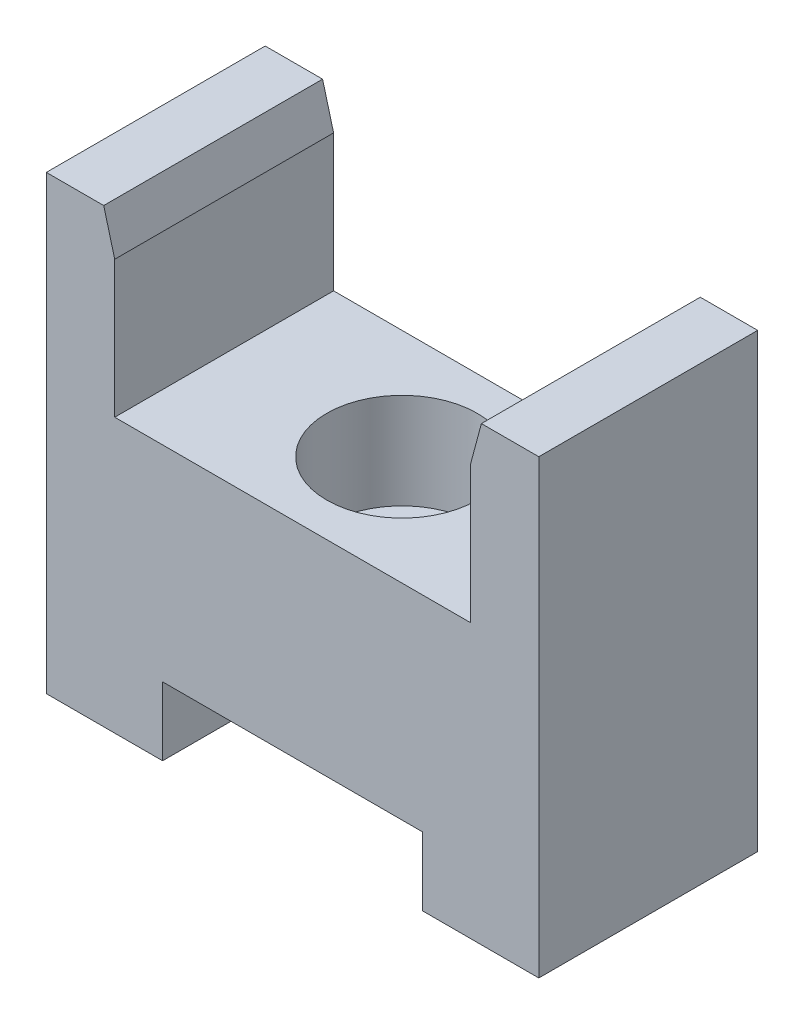
SolidWorks part; units mm, degrees
material "AISI 1045 钢，冷拔"
ref_plane "Front Plane" through (0, 0, 0) normal (0, 0, 1) x (1, 0, 0)
ref_plane "Top Plane" through (0, 0, 0) normal (0, 1, 0) x (1, 0, 0)
ref_plane "Right Plane" through (0, 0, 0) normal (1, 0, 0) x (0, 0, -1)
sketch "Sketch1" plane through (0, 0, 0) normal (0, 0, 1) x (1, 0, 0)
  line L0 (0, 33) -> (0, 0)
  line L1 (0, 0) -> (8.5, 0)
  line L2 (8.5, 0) -> (8.5, 5)
  line L3 (8.5, 5) -> (27.5, 5)
  line L4 (27.5, 5) -> (27.5, 0)
  line L5 (27.5, 0) -> (36, 0)
  line L6 (36, 0) -> (36, 33)
  line L10 (0, 33) -> (4.1962, 33)
  line L11 (4.1962, 33) -> (5, 30)
  line L12 (5, 30) -> (5, 20)
  line L13 (5, 20) -> (31, 20)
  line L14 (31, 20) -> (31, 30)
  line L15 (31, 30) -> (31.8038, 33)
  line L16 (31.8038, 33) -> (36, 33)
  dimension "D1" = 33
  dimension "D2" = 8.5
  dimension "D3" = 19
  dimension "D4" = 8.5
  dimension "D5" = 13
  dimension "D6" = 13
  dimension "D7" = 26
  dimension "D8" = 3
  dimension "D9" = 105
  dimension "D10" = 3
  dimension "D11" = 105
  dimension "D12" = 5
  dimension "D13" = 5
extrude "Boss-Extrude1" add sketch "Sketch1" along normal blind 16
ref_plane "Plane1" through (0, 20, 0) normal (0, 1, 0) x (1, 0, 0)
sketch "Sketch2" plane through (0, 20, 0) normal (0, 1, 0) x (1, 0, 0)
  circle A0 centre (18, -8) radius 5.5
extrude "Cut-Extrude1" cut sketch "Sketch2" against normal blind 7
ref_plane "Plane2" through (0, 13, 0) normal (0, 1, 0) x (1, 0, 0)
sketch "Sketch3" plane through (0, 13, 0) normal (0, 1, 0) x (1, 0, 0)
  circle A0 centre (18, -8) radius 3.5
extrude "Cut-Extrude2" cut sketch "Sketch3" against normal blind 8
